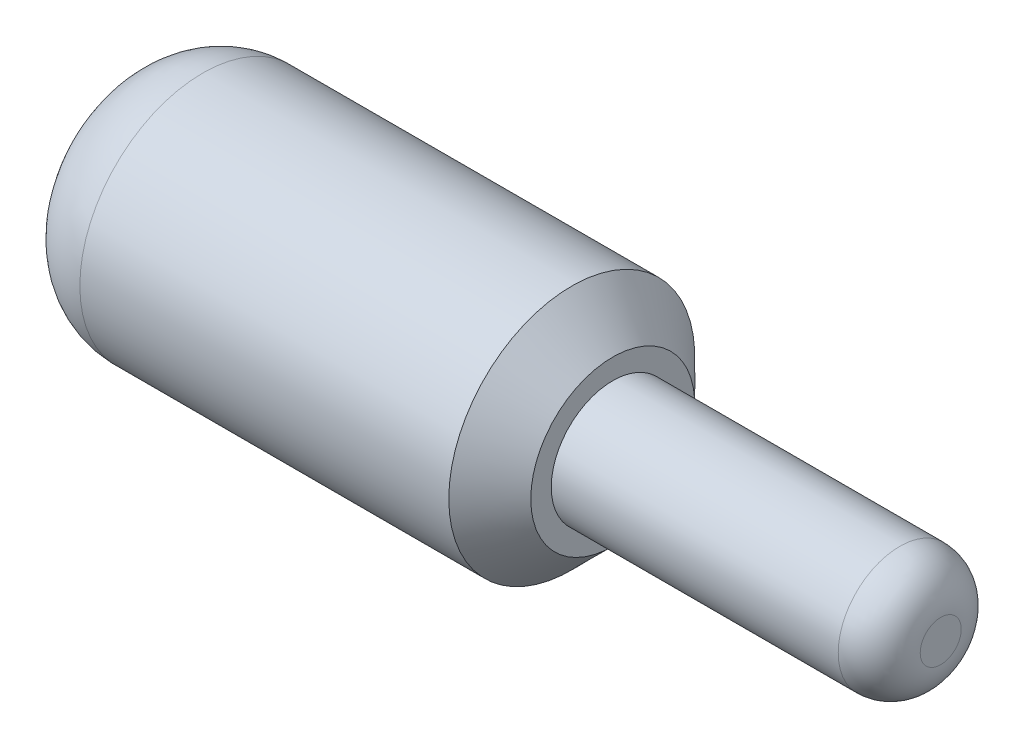
from build123d import *

# Parameters (mm, degrees)
FILLET1_R     = 2
FILLET2_R     = 1
CHAMFER1_SIZE = 1


with BuildPart() as part:
    # Sketch1 → Revolve1 (revolve)
    with BuildSketch(Plane.XY, mode=Mode.PRIVATE) as revolve1_sk:
        Polygon((0, 0), (0, 3), (12, 3), (12, 1.5), (20, 1.5), (20, 0), align=None)
    revolve(revolve1_sk.sketch.rotate(Axis((0, 0, 0), (1, 0, 0)), 90), axis=Axis((0, 0, 0), (1, 0, 0)))

    # Fillet1
    fillet1_edges = [part.edges().sort_by_distance(p)[0] for p in [
        (0, 0, -3),
    ]]
    fillet(fillet1_edges, radius=FILLET1_R)

    # Fillet2
    fillet2_edges = [part.edges().sort_by_distance(p)[0] for p in [
        (20, 0, -1.5),
    ]]
    fillet(fillet2_edges, radius=FILLET2_R)

    # Chamfer1
    chamfer1_edges = [part.edges().sort_by_distance(p)[0] for p in [
        (12, 0, -3),
    ]]
    chamfer(chamfer1_edges, length=CHAMFER1_SIZE)


solid = part.part
